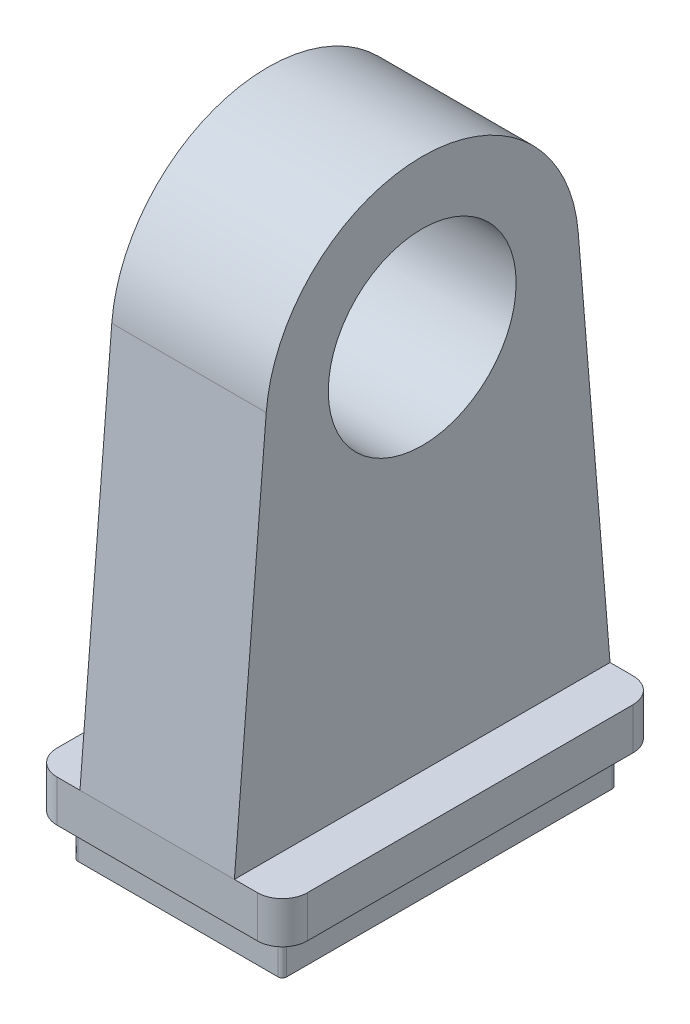
from build123d import *

# Parameters (mm, degrees)
BOSS_EXTRUDE_1_DEPTH = 20
BOSS_EXTRUDE_2_DEPTH = 20
SKETCH_3_R           = 45
BOSS_EXTRUDE_3_DEPTH = 37


with BuildPart() as part:
    # Sketch 1 → Boss-Extrude 1 (new body)
    with BuildSketch(Plane(origin=(0, 0, 0), x_dir=(1, 0, 0), z_dir=(0, 1, 0))):
        with BuildLine():
            Line((48, 90), (-48, 90))
            ThreePointArc((-48, 90), (-56.485281374, 86.485281374), (-60, 78))
            Line((-60, 78), (-60, -78))
            ThreePointArc((-60, -78), (-56.485281374, -86.485281374), (-48, -90))
            Line((-48, -90), (48, -90))
            ThreePointArc((48, -90), (56.485281374, -86.485281374), (60, -78))
            Line((60, -78), (60, 78))
            ThreePointArc((60, 78), (56.485281374, 86.485281374), (48, 90))
        make_face()
    extrude(amount=BOSS_EXTRUDE_1_DEPTH)

    # Sketch 2 → Boss-Extrude 2 (add)
    with BuildSketch(Plane.XZ):
        with BuildLine():
            Line((-48, -80), (48, -80))
            ThreePointArc((48, -80), (49.414213562, -79.414213562), (50, -78))
            Line((50, -78), (50, 78))
            ThreePointArc((50, 78), (49.414213562, 79.414213562), (48, 80))
            Line((48, 80), (-48, 80))
            ThreePointArc((-48, 80), (-49.414213562, 79.414213562), (-50, 78))
            Line((-50, 78), (-50, -78))
            ThreePointArc((-50, -78), (-49.414213562, -79.414213562), (-48, -80))
        make_face()
    extrude(amount=BOSS_EXTRUDE_2_DEPTH)

    # Sketch 3 → Boss-Extrude 3 (add, symmetric)
    with BuildSketch(Plane(origin=(0, 0, 0), x_dir=(0, 0, -1), z_dir=(1, 0, 0))):
        with BuildLine():
            Line((-74.74949799, 206.124748995), (-90, 20))
            Line((-90, 20), (90, 20))
            Line((90, 20), (74.74949799, 206.124748995))
            ThreePointArc((74.74949799, 206.124748995), (0, 275), (-74.74949799, 206.124748995))
        make_face()
        with Locations((0, 200)):
            Circle(SKETCH_3_R, mode=Mode.SUBTRACT)
    extrude(amount=BOSS_EXTRUDE_3_DEPTH, both=True)


solid = part.part
